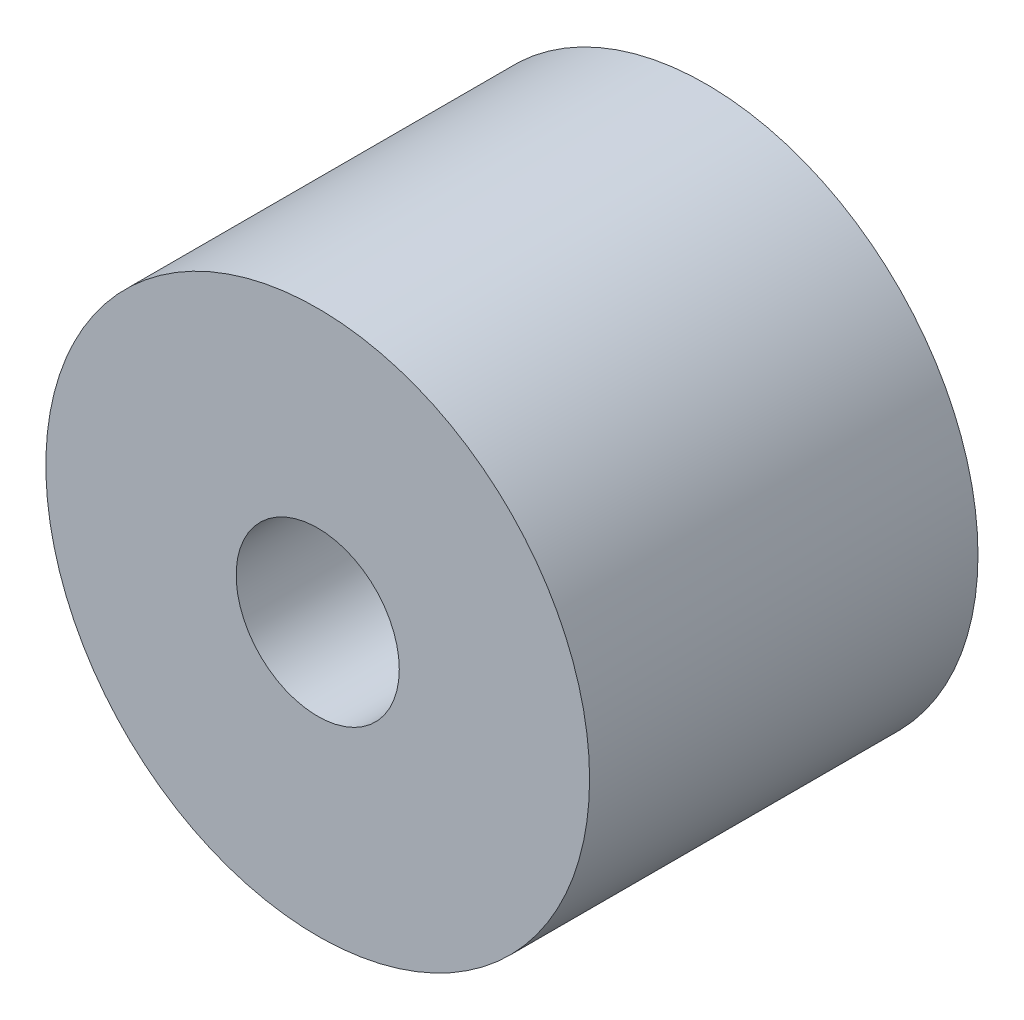
SolidWorks part; units mm, degrees
ref_plane "前视基准面" through (0, 0, 0) normal (0, 0, 1) x (1, 0, 0)
ref_plane "上视基准面" through (0, 0, 0) normal (0, 1, 0) x (1, 0, 0)
ref_plane "右视基准面" through (0, 0, 0) normal (1, 0, 0) x (0, 0, -1)
sketch "草图1" plane through (0, 0, 0) normal (0, 0, 1) x (1, 0, 0)
  circle A0 centre (0, 0) radius 7
  dimension "D1" = 14
extrude "凸台-拉伸1" add sketch "草图1" along normal blind 10
hole_wizard "M5 螺纹孔1" positions "草图3" profile "草图4" tap size "M5" standard "Iso" end condition through all
sketch "草图3" plane through (0, 0, 10) normal (0, 0, 1) x (1, 0, 0)
  point P0 (0, 0)
sketch "草图4" plane through (0, 0, 10) normal (1, 0, 0) x (0, -1, 0)
  line L0 (0, 0) -> (0, 10)
  line L1 (0, 10) -> (2.1, 10)
  line L2 (2.1, 10) -> (2.1, 0)
  line L5 (2.1, 0) -> (0, 0)
  line L11 (0, -6.35) -> (0, 107.95) construction
  dimension "通孔螺纹孔钻头直径" = 4.2
  dimension "通孔螺纹孔钻头深度" = 10
cosmetic thread "孔螺蚊线1" parameters "D2"=5
